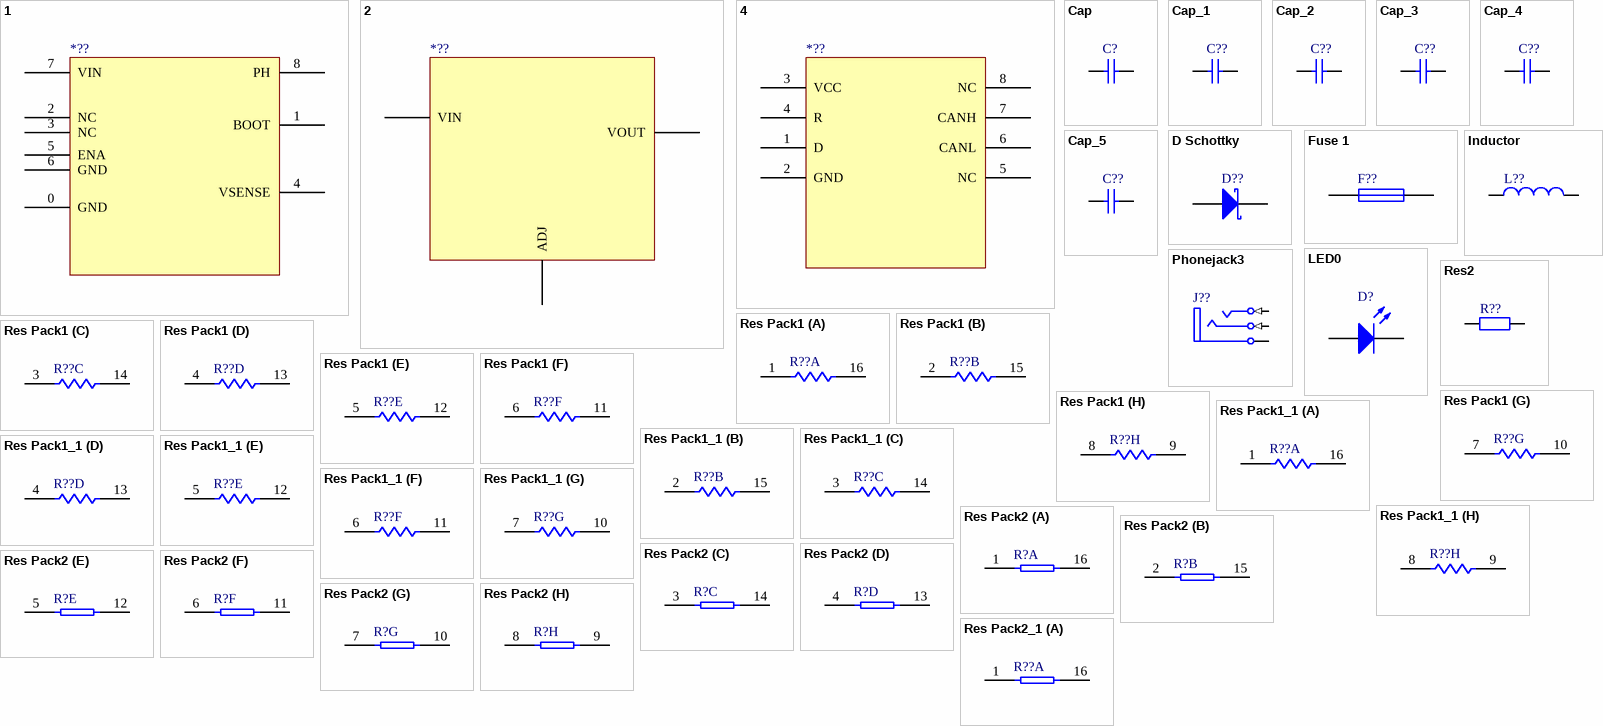
[diagram p0: symbols 1 to Res Pack2_1]
# Altium schematic symbol library MISC82341-11.SCHLIB: 26 symbols
Pins are listed as number, name and electrical type; pins without a type are passive.


## 1
designator *??
pins: 0 GND, 1 BOOT, 2 NC, 3 NC, 4 VSENSE, 5 ENA, 6 GND, 7 VIN, 8 PH

## 2
designator *??
pins: ?1 VIN, ?2 ADJ, ?3 VOUT

## 4
designator *??
pins: 1 D, 2 GND, 3 VCC, 4 R, 5 NC, 6 CANL, 7 CANH, 8 NC

## Cap
designator C?
Capacitor
footprint RAD-0.3 (Radial Cap, Thru-Hole; 2 Leads; 0.3 in Pin Spacing)
simulation model CAP (Capacitor)
signal-integrity model Cap
pins: 1, 2

## Cap_1
designator C??
Capacitor
footprint RAD-0.3 (Radial Cap, Thru-Hole; 2 Leads; 0.3 in Pin Spacing)
simulation model CAP (Capacitor)
signal-integrity model Cap
pins: 1, 2

## Cap_2
designator C??
Capacitor
footprint RAD-0.3 (Radial Cap, Thru-Hole; 2 Leads; 0.3 in Pin Spacing)
simulation model CAP (Capacitor)
signal-integrity model Cap
pins: 1, 2

## Cap_3
designator C??
Capacitor
footprint RAD-0.3 (Radial Cap, Thru-Hole; 2 Leads; 0.3 in Pin Spacing)
simulation model CAP (Capacitor)
signal-integrity model Cap
pins: 1, 2

## Cap_4
designator C??
Capacitor
footprint RAD-0.3 (Radial Cap, Thru-Hole; 2 Leads; 0.3 in Pin Spacing)
simulation model CAP (Capacitor)
signal-integrity model Cap
pins: 1, 2

## Cap_5
designator C??
Capacitor
footprint RAD-0.3 (Radial Cap, Thru-Hole; 2 Leads; 0.3 in Pin Spacing)
simulation model CAP (Capacitor)
signal-integrity model Cap
pins: 1, 2

## D Schottky
designator D??
Schottky Diode
footprint SMB (DO-214-AA/SMB; 2 C-Bend Leads; Body 5.3 x 3.6 mm, inc. leads (LxW))
simulation model SKYDIODE (Diode)
signal-integrity model D Schottky
pins: 1 A, 2 K

## Fuse 1
designator F??
Fuse
footprint PIN-W2/E2.8 (Thru-Hole; 2 Leads)
simulation model FUSE (Spice Subcircuit)
pins: 1, 2

## Inductor
designator L??
Inductor
footprint 0402-A (Chip Inductor, Body 1.0x0.5mm, IPC High Density)
footprint INDC1608L (Chip Inductor, Body 1.6x0.8mm, IPC High Density)
footprint 2029 (Chip Inductor, Body 2.0x1.2mm, IPC High Density)
footprint 0603 (Chip Inductor, Body 0.6x0.3mm, IPC High Density)
footprint INDC3216 (Chip Inductor, Body 3.2x1.6mm, IPC High Density)
footprint INDC4532 (Chip Inductor, Body 4.5x3.2mm, IPC High Density)
simulation model INDUCTOR (Inductor)
signal-integrity model Inductor
pins: 1, 2

## LED0
designator D?
Typical INFRARED GaAs LED
footprint LED-0 (LED; 2 Leads)
simulation model LED0 (Diode)
pins: 1 A, 2 K

## Phonejack3
designator J??
Jack Socket, 1/4" [6.5mm], Thru-Hole, Vertical, 3-Conductor Open Circuit (Non-Normalling)
footprint JACK/6-V3 (Connector; Jack Socket, 1/4" [6.5mm], Thru-Hole, 3 Position, Vertical, Body 15.7 x 15.7 x 31 mm (WxTxH))
signal-integrity model JACK Socket
pins: 1 T (in) "Tip/Left Channel/(+)", 3 R (in) "Ring/Right Channel/(-)", 5 S (power) "Sleeve (Ground)"

## Res2
designator R??
Resistor
footprint AXIAL-0.4 (Axial Device, Thru-Hole; 2 Leads; 0.4 in Pin Spacing)
simulation model RESISTOR (Resistor)
signal-integrity model Res
pins: 1, 2

## Res Pack1
designator R??
Isolated Resistor Network - Parts
footprint SOIC16_N (SOIC, 16-Leads, Body 9.9x3.9mm, Pitch 1.27mm, IPC Medium Density)
footprint SOIC16_L (SOIC, 16-Leads, Body 9.9x3.9mm, Pitch 1.27mm, IPC High Density)
footprint SOIC16_M (SOIC, 16-Leads, Body 9.9x3.9mm, Pitch 1.27mm, IPC Low Density)
simulation model RESISTOR (Resistor)
signal-integrity model Res Pack
part A pins: 1, 16
part B pins: 2, 15
part C pins: 3, 14
part D pins: 4, 13
part E pins: 5, 12
part F pins: 6, 11
part G pins: 7, 10
part H pins: 8, 9

## Res Pack1_1
designator R??
Isolated Resistor Network - Parts
footprint SOIC16_N (SOIC, 16-Leads, Body 9.9x3.9mm, Pitch 1.27mm, IPC Medium Density)
footprint SOIC16_L (SOIC, 16-Leads, Body 9.9x3.9mm, Pitch 1.27mm, IPC High Density)
footprint SOIC16_M (SOIC, 16-Leads, Body 9.9x3.9mm, Pitch 1.27mm, IPC Low Density)
simulation model RESISTOR (Resistor)
signal-integrity model Res Pack
part A pins: 1, 16
part B pins: 2, 15
part C pins: 3, 14
part D pins: 4, 13
part E pins: 5, 12
part F pins: 6, 11
part G pins: 7, 10
part H pins: 8, 9

## Res Pack2
designator R?
Isolated Resistor Network - Parts
footprint DIP-16 (DIP; 16 Leads; Row Spacing 7.62 mm; Pitch 2.54 mm)
simulation model RESISTOR (Resistor)
signal-integrity model Res Pack
part A pins: 1, 16
part B pins: 2, 15
part C pins: 3, 14
part D pins: 4, 13
part E pins: 5, 12
part F pins: 6, 11
part G pins: 7, 10
part H pins: 8, 9

## Res Pack2_1
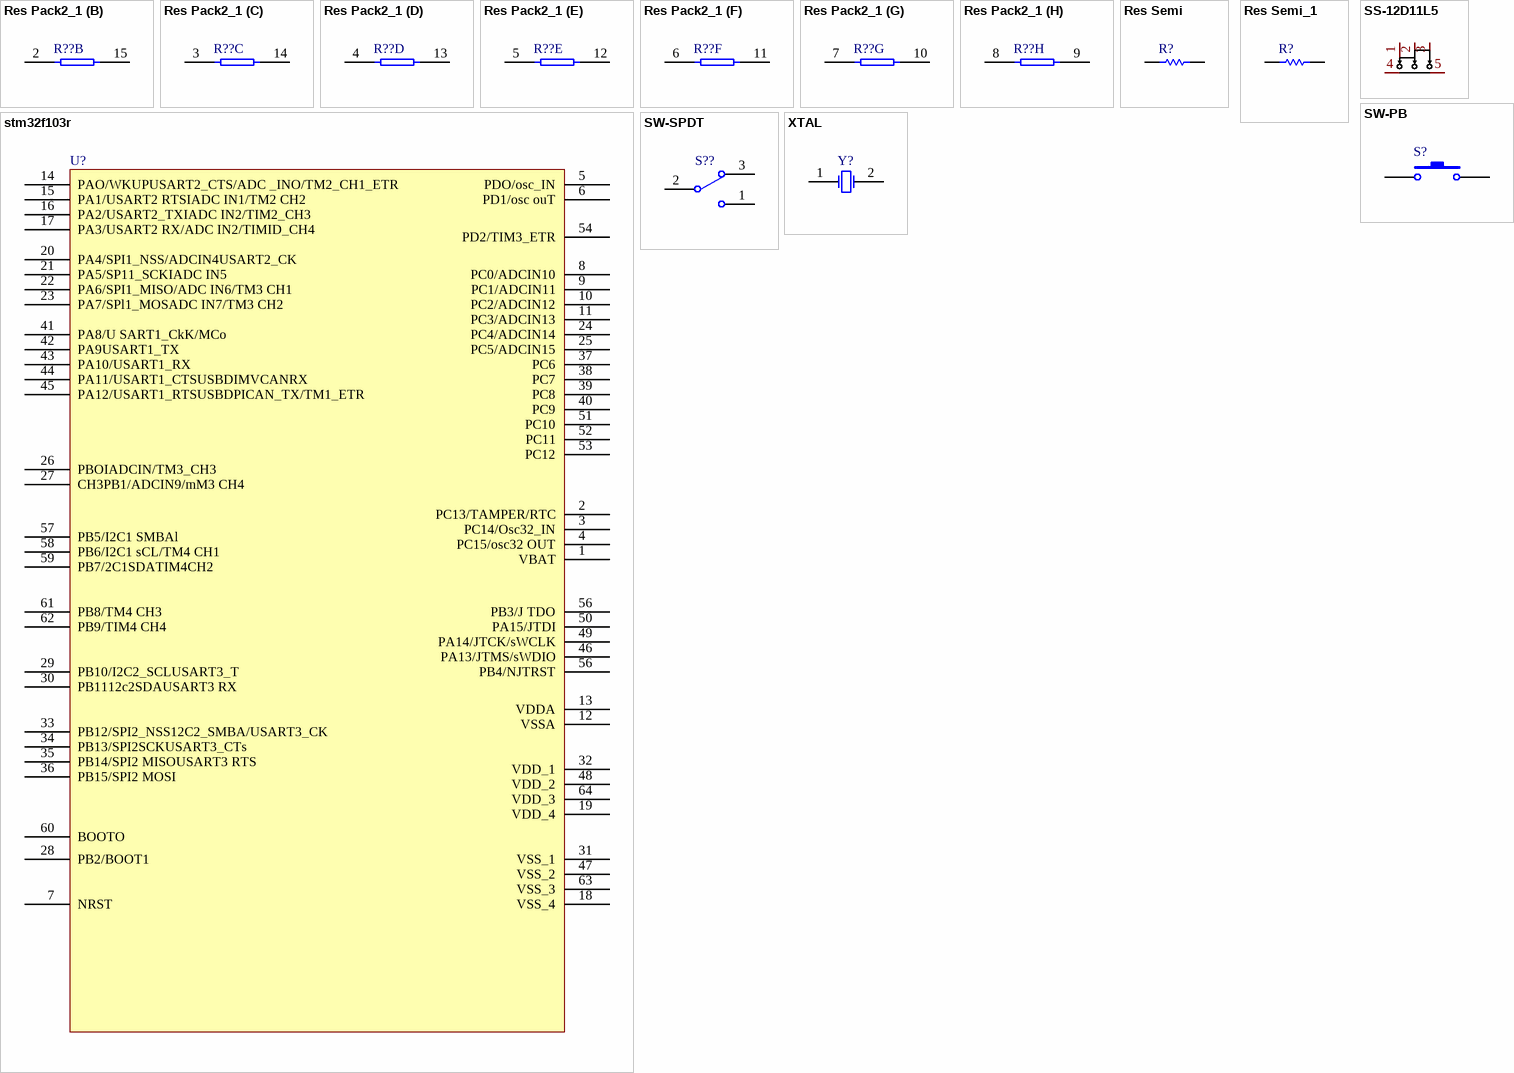
[diagram p1: symbols Res Pack2_1 to XTAL]
## Res Pack2_1
designator R??
Isolated Resistor Network - Parts
footprint DIP-16 (DIP; 16 Leads; Row Spacing 7.62 mm; Pitch 2.54 mm)
simulation model RESISTOR (Resistor)
signal-integrity model Res Pack
part A pins: 1, 16
part B pins: 2, 15
part C pins: 3, 14
part D pins: 4, 13
part E pins: 5, 12
part F pins: 6, 11
part G pins: 7, 10
part H pins: 8, 9

## Res Semi
designator R?
Semiconductor Resistor
footprint AXIAL-0.5 (Axial Device, Thru-Hole; 2 Leads; 0.5 in Pin Spacing)
simulation model RES (Semiconductor Resistor)
signal-integrity model Res Semi
pins: 1, 2

## Res Semi_1
designator R?
Semiconductor Resistor
footprint AXIAL-0.5 (Axial Device, Thru-Hole; 2 Leads; 0.5 in Pin Spacing)
simulation model RES (Semiconductor Resistor)
signal-integrity model Res Semi
pins: 1, 2

## SS-12D11L5
designator SW??
footprint SW-TH_SS-12D11L5
3D model SW-TH_SS-12D11L5
pins: 1, 2, 3, 4, 5

## stm32f103r
designator U?
pins: 1 VBAT, 2 PC13/TAMPER/RTC, 3 PC14/Osc32_IN, 4 PC15/osc32 OUT, 5 PDO/osc_IN, 6 PD1/osc ouT, 7 NRST, 8 PC0/ADCIN10, 9 PC1/ADCIN11, 10 PC2/ADCIN12, 11 PC3/ADCIN13, 12 VSSA, 13 VDDA, 14 PAO/WKUPUSART2_CTS/ADC _INO/TM2_CH1_ETR, 15 PA1/USART2 RTSIADC IN1/TM2 CH2, 16 PA2/USART2_TXIADC IN2/TIM2_CH3, 17 PA3/USART2 RX/ADC IN2/TIMID_CH4, 18 VSS_4, 19 VDD_4, 20 PA4/SPI1_NSS/ADCIN4USART2_CK, 21 PA5/SP11_SCKIADC IN5, 22 PA6/SPI1_MISO/ADC IN6/TM3 CH1, 23 PA7/SPl1_MOSADC IN7/TM3 CH2, 24 PC4/ADCIN14, 25 PC5/ADCIN15, 26 PBOIADCIN/TM3_CH3, 27 CH3PB1/ADCIN9/mM3 CH4, 28 PB2/BOOT1, 29 PB10/I2C2_SCLUSART3_T, 30 PB1112c2SDAUSART3 RX, 31 VSS_1, 32 VDD_1, 33 PB12/SPI2_NSS12C2_SMBA/USART3_CK, 34 PB13/SPI2SCKUSART3_CTs, 35 PB14/SPI2 MISOUSART3 RTS, 36 PB15/SPI2 MOSI, 37 PC6, 38 PC7, 39 PC8, 40 PC9, 41 PA8/U SART1_CkK/MCo, 42 PA9USART1_TX, 43 PA10/USART1_RX, 44 PA11/USART1_CTSUSBDIMVCANRX, 45 PA12/USART1_RTSUSBDPICAN_TX/TM1_ETR, 46 PA13/JTMS/sWDIO, 47 VSS_2, 48 VDD_2, 49 PA14/JTCK/sWCLK, 50 PA15/JTDI, 51 PC10, 52 PC11, 53 PC12, 54 PD2/TIM3_ETR, 56 PB3/J TDO, 56 PB4/NJTRST, 57 PB5/I2C1 SMBAl, 58 PB6/I2C1 sCL/TM4 CH1, 59 PB7/2C1SDATIM4CH2, 60 BOOTO, 61 PB8/TM4 CH3, 62 PB9/TIM4 CH4, 63 VSS_3, 64 VDD_3

## SW-PB
designator S?
Switch
footprint SPST-2 (Switch; 2 Leads)
pins: 1, 2

## SW-SPDT
designator S??
SPDT Subminiature Toggle Switch, Right Angle Mounting, Vertical Actuation
footprint TL36WW15050 (Switch; 4 Leads)
pins: 1, 2, 3

## XTAL
designator Y?
Crystal Oscillator
footprint R38 (Crystal, Thru-Hole; 2 Leads; Body 3.1 x 8.2 mm (Dia.xH))
simulation model XTAL (Spice Subcircuit)
pins: 1 OSC1, 2 OSC2